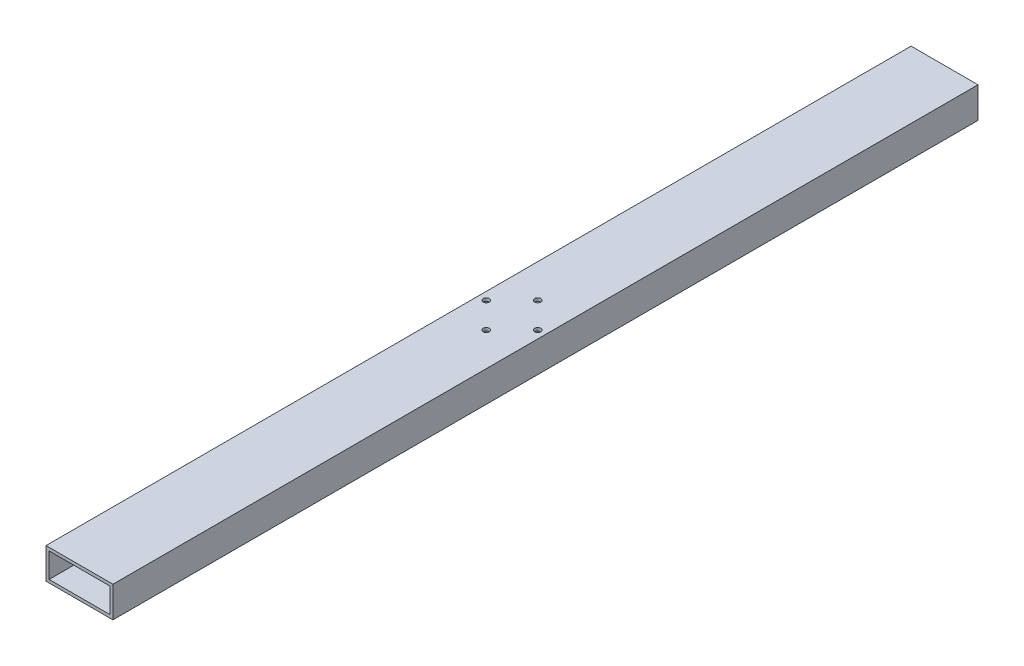
from build123d import *

# Parameters (mm, degrees)
SKETCH1_W           = 65
SKETCH1_H           = 30
BOSS_EXTRUDE1_DEPTH = 840
SKETCH2_W           = 59
SKETCH2_H           = 24
CUT_EXTRUDE1_DEPTH  = 950
SKETCH5_R           = 3
CUT_EXTRUDE3_DEPTH  = 842.512657385


with BuildPart() as part:
    # Sketch1 → Boss-Extrude1 (new body)
    with BuildSketch(Plane.XY):
        with Locations((-8.040751589, 24.808027615)):
            Rectangle(SKETCH1_W, SKETCH1_H)
    extrude(amount=BOSS_EXTRUDE1_DEPTH)

    # Sketch2 → Cut-Extrude1 (cut)
    with BuildSketch(Plane.XY.offset(840)):
        with Locations((-8.040751589, 24.808027615)):
            Rectangle(SKETCH2_W, SKETCH2_H)
    extrude(amount=-CUT_EXTRUDE1_DEPTH, mode=Mode.SUBTRACT)

    # Sketch5 → Cut-Extrude3 (cut, through all)
    with BuildSketch(Plane(origin=(0, 9.808027615, 0), x_dir=(-1, 0, 0), z_dir=(0, -1, 0))):
        with Locations(Location((8.040751589, -395, 0), (0, 0, 90))):
            Circle(SKETCH5_R)
        with Locations(Location((33.040751589, -420, 0), (0, 0, 90))):
            Circle(SKETCH5_R)
        with Locations(Location((8.040751589, -445, 0), (0, 0, 90))):
            Circle(SKETCH5_R)
        with Locations(Location((-16.959248411, -420, 0), (0, 0, 90))):
            Circle(SKETCH5_R)
    extrude(amount=-CUT_EXTRUDE3_DEPTH, mode=Mode.SUBTRACT)


solid = part.part
